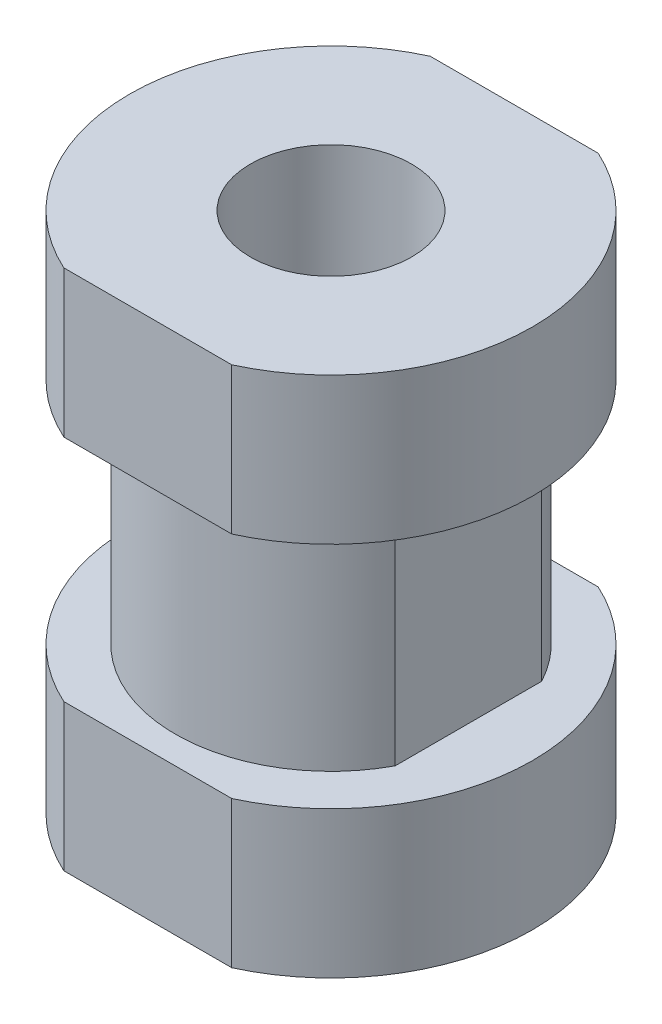
SolidWorks part; units mm, degrees
material "AISI 304"
ref_plane "前视基准面" through (0, 0, 0) normal (0, 0, 1) x (1, 0, 0)
ref_plane "上视基准面" through (0, 0, 0) normal (0, 1, 0) x (1, 0, 0)
ref_plane "右视基准面" through (0, 0, 0) normal (1, 0, 0) x (0, 0, -1)
sketch "草图1" plane through (0, 0, 0) normal (0, 1, 0) x (1, 0, 0)
  circle A0 centre (0, 0) radius 11
  dimension "D1" = 22
extrude "凸台-拉伸1" add sketch "草图1" along normal mid plane 8
sketch "草图2" plane through (0, 4, 0) normal (0, 1, 0) x (1, 0, 0)
  circle A0 centre (0, 0) radius 8.5
  dimension "D1" = 17
extrude "凸台-拉伸2" add sketch "草图2" along normal blind 12.5
sketch "草图9" plane through (0, 16.5, 0) normal (0, 1, 0) x (1, 0, 0)
  circle A1 centre (0, 0) radius 11 construction
  circle A2 centre (0, 0) radius 11
extrude "凸台-拉伸3" add sketch "草图9" along normal blind 8
sketch "草图3" plane through (0, -4, 0) normal (0, -1, 0) x (-1, 0, 0)
  point P0 (0, 0)
hole_wizard "M10x1.25 螺纹孔1" positions "草图3" profile "草图4" tap size "M10x1.25" standard "ISO" end condition through all
sketch "草图4" plane through (0, -4, 0) normal (1, 0, 0) x (0, 0, -1)
  line L0 (0, 0) -> (0, 28.5)
  line L1 (0, 28.5) -> (4.4, 28.5)
  line L2 (4.4, 28.5) -> (4.4, 0)
  line L5 (4.4, 0) -> (0, 0)
  line L11 (0, -6.35) -> (0, 107.95) construction
  dimension "通孔螺纹孔钻头直径" = 8.8
  dimension "通孔螺纹孔钻头深度" = 28.5
sketch "草图5" plane through (0, -4, 0) normal (0, -1, 0) x (1, 0, 0)
  line L1 (-11, 9) -> (11, 9)
  line L2 (-11, 9) -> (-11, -9)
  line L3 (-11, -9) -> (11, -9)
  line L4 (11, 9) -> (11, -9)
  line L5 (-11, 9) -> (11, -9) construction
  line L6 (-11, -9) -> (11, 9) construction
  circle A0 centre (0, 0) radius 11 construction
  point P0 (0, 0)
  dimension "D1" = 2
extrude "切除-拉伸1" [suppressed] cut sketch "草图5" against normal through all both and the other way through all flip side to cut
sketch "草图6" plane through (0, -4, 0) normal (0, -1, 0) x (1, 0, 0)
  line L1 (0, 0) -> (0, -11) construction
  line L3 (-4.5826, 10) -> (4.5826, 10)
  line L4 (0, 0) -> (0, 10) construction
  line L5 (-4.5826, -10) -> (4.5826, -10)
  circle A0 centre (0, 0) radius 11 construction
  circle A3 centre (0, 0) radius 11 construction
  arc A4 (-4.5826, -10) -> (4.5826, -10) centre (0, 0) ccw
  arc A5 (4.5826, 10) -> (-4.5826, 10) centre (0, 0) ccw
  dimension "D1" = 20
extrude "切除-拉伸2" cut sketch "草图6" against normal through all
sketch "草图10" plane through (0, 0, 0) normal (0, 0, 1) x (1, 0, 0)
  line L0 (-8.5, 16.5) -> (8.5, 16.5) construction
  line L1 (-8.5, 4) -> (-7.5, 4)
  line L2 (-8.5, 4) -> (-8.5, 16.5)
  line L3 (-8.5, 16.5) -> (-7.5, 16.5)
  line L4 (-7.5, 4) -> (-7.5, 16.5)
  line L5 (0, 24.5) -> (0, -4) construction
  line L6 (4.5826, 24.5) -> (-4.5826, 24.5) construction
  line L7 (4.5826, -4) -> (-4.5826, -4) construction
  line L8 (7.5, 4) -> (7.5, 16.5)
  line L9 (8.5, 16.5) -> (7.5, 16.5)
  line L10 (8.5, 4) -> (8.5, 16.5)
  line L11 (8.5, 4) -> (7.5, 4)
  dimension "D1" = 15
extrude "切除-拉伸3" cut sketch "草图10" against normal mid plane 49
